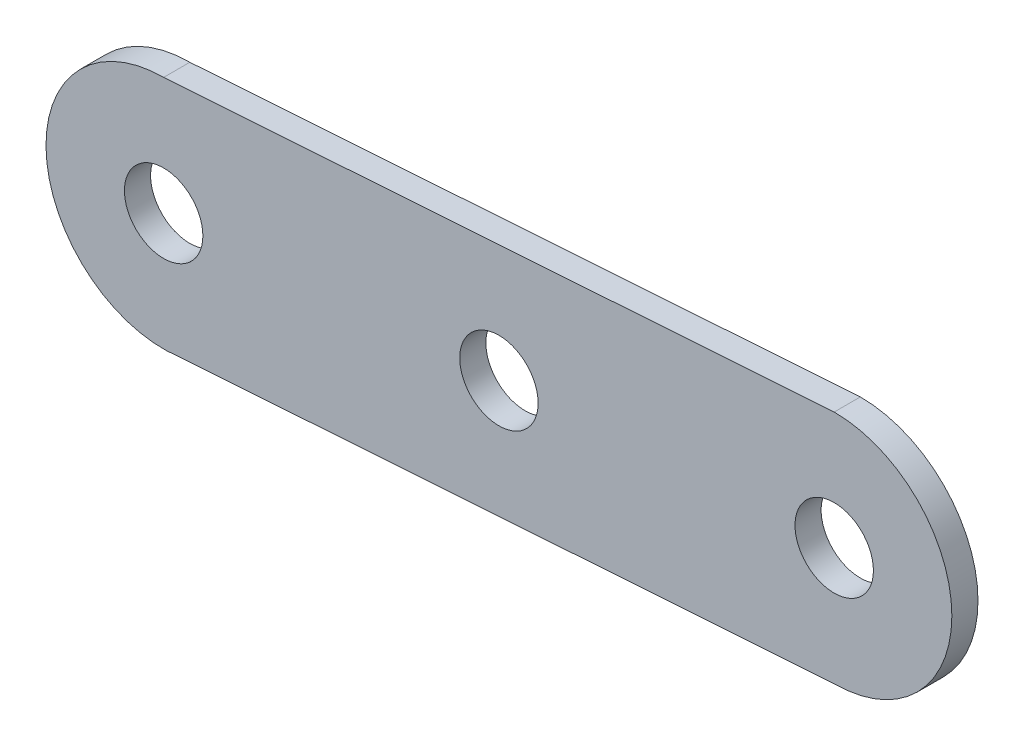
from build123d import *

# Parameters (mm, degrees)
SKETCH1_R           = 3
BOSS_EXTRUDE1_DEPTH = 2


with BuildPart() as part:
    # Sketch1 → Boss-Extrude1 (new body)
    with BuildSketch(Plane.XY):
        with BuildLine():
            Line((-51.293623615, 5.521870404), (0, 9))
            ThreePointArc((0, 9), (9, 0), (0, -9))
            Line((0, -9), (-50.078661895, -12.395745198))
            ThreePointArc((-50.078661895, -12.395745198), (-60.273003894, -4.087005439), (-51.293623615, 5.521870404))
        make_face()
        with Locations((-51.293623615, -3.478129596)):
            Circle(SKETCH1_R, mode=Mode.SUBTRACT)
        Circle(SKETCH1_R, mode=Mode.SUBTRACT)
        with Locations((-25.646811807, -1.739064798)):
            Circle(SKETCH1_R, mode=Mode.SUBTRACT)
    extrude(amount=BOSS_EXTRUDE1_DEPTH)


solid = part.part
